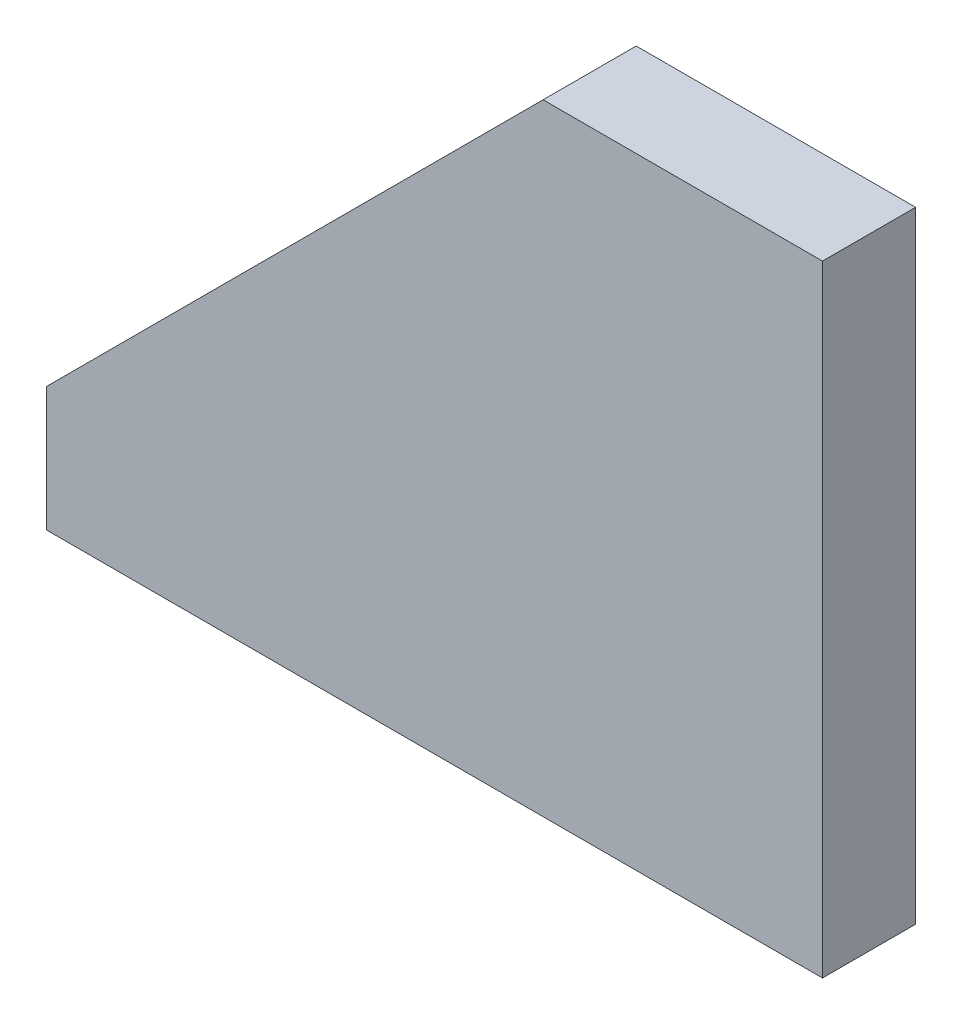
SolidWorks part; units mm, degrees
material "A6061"
ref_plane "前视基准面" through (0, 0, 0) normal (0, 0, 1) x (1, 0, 0)
ref_plane "上视基准面" through (0, 0, 0) normal (0, 1, 0) x (1, 0, 0)
ref_plane "右视基准面" through (0, 0, 0) normal (1, 0, 0) x (0, 0, -1)
sketch "草图1" plane through (0, 0, 0) normal (0, 0, 1) x (1, 0, 0)
  line L1 (-62.5, -50) -> (62.5, -50)
  line L2 (-62.5, -50) -> (-62.5, 50)
  line L3 (-62.5, 50) -> (62.5, 50)
  line L4 (62.5, -50) -> (62.5, 50)
  line L5 (-62.5, -50) -> (62.5, 50) construction
  line L6 (-62.5, 50) -> (62.5, -50) construction
  point P0 (0, 0)
  dimension "D1" = 125
  dimension "D2" = 100
extrude "凸台-拉伸1" add sketch "草图1" along normal blind 15
chamfer "倒角1" distance 80 angle 45 1 edges at (-62.5, 50, 7.5)
